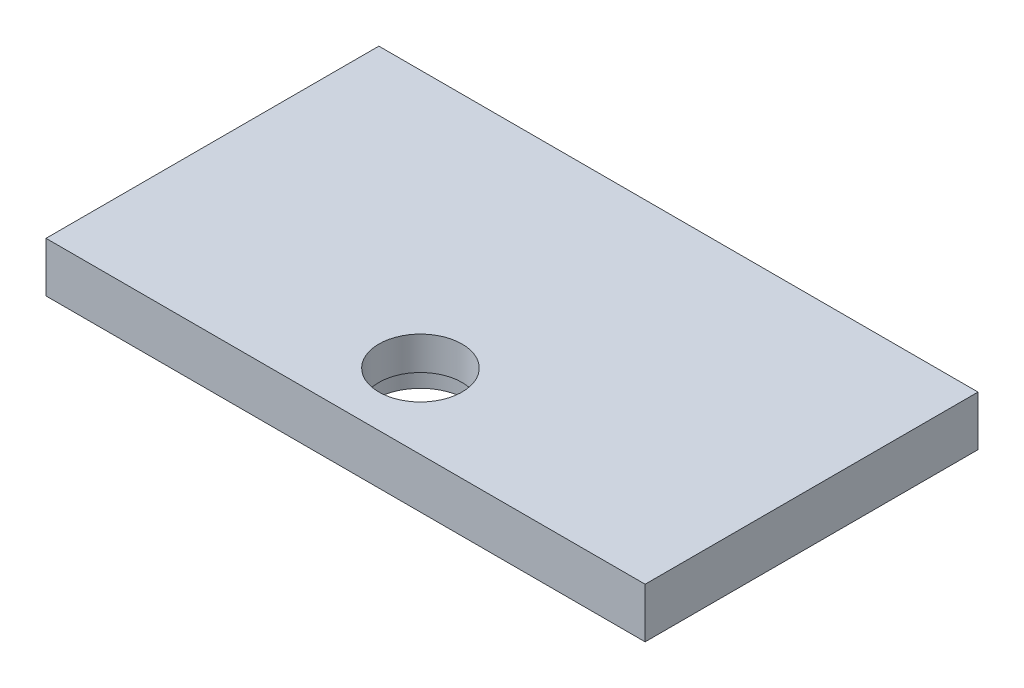
from build123d import *

# Parameters (mm, degrees)
SKETCH_1_W          = 360
SKETCH_1_H          = 200
EXTRUDE_1_DEPTH     = 30
SKETCH_2_R          = 25
CUT_EXTRUDE_1_DEPTH = 209.086520467
SKETCH_3_R          = 27.5
CUT_EXTRUDE_2_DEPTH = 10


with BuildPart() as part:
    # 草图1 → 凸台-拉伸1 (new body)
    with BuildSketch(Plane(origin=(0, 0, 0), x_dir=(1, 0, 0), z_dir=(0, 1, 0))):
        Rectangle(SKETCH_1_W, SKETCH_1_H)
    extrude(amount=EXTRUDE_1_DEPTH)

    # 草图2 → 切除-拉伸1 (cut, through all)
    with BuildSketch(Plane.XZ):
        with Locations(Location((0, 55, 0), (0, 0, 270))):
            Circle(SKETCH_2_R)
    extrude(amount=-CUT_EXTRUDE_1_DEPTH, mode=Mode.SUBTRACT)

    # 草图3 → 切除-拉伸2 (cut)
    with BuildSketch(Plane.XZ):
        with Locations(Location((0, 55, 0), (0, 0, 270))):
            Circle(SKETCH_3_R)
    extrude(amount=-CUT_EXTRUDE_2_DEPTH, mode=Mode.SUBTRACT)


solid = part.part
